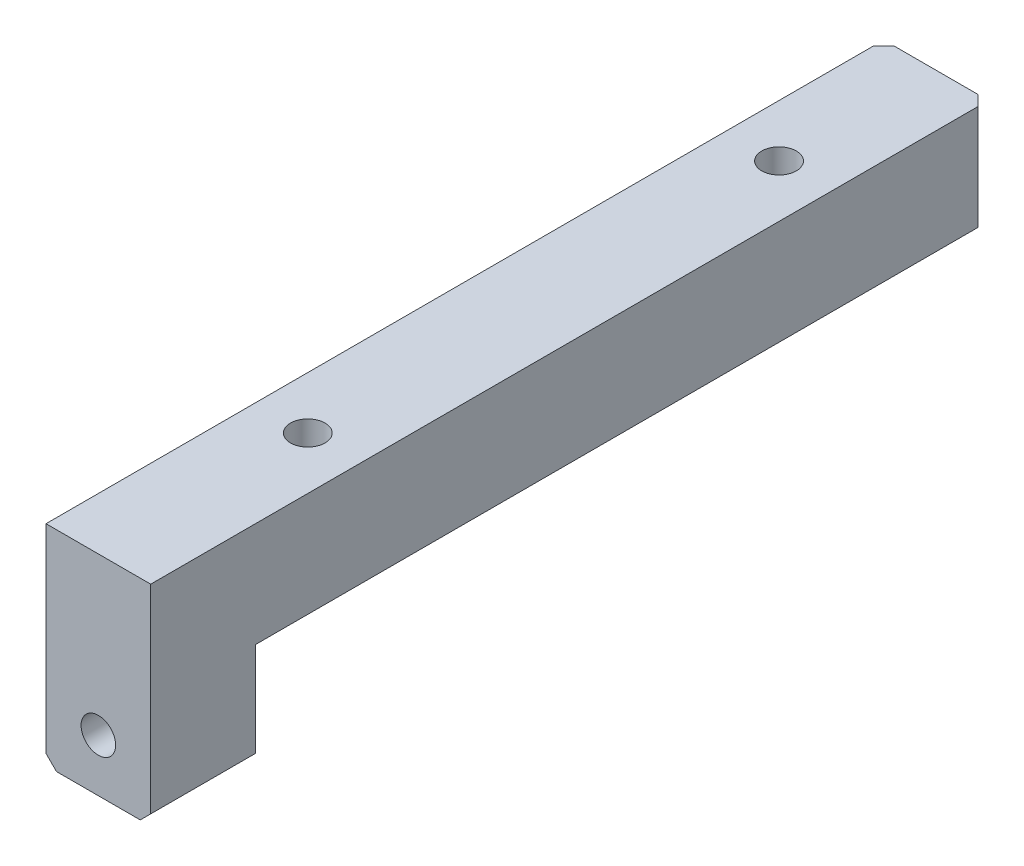
SolidWorks part; units mm, degrees
material "AL6061"
ref_plane "Front Plane" through (0, 0, 0) normal (0, 0, 1) x (1, 0, 0)
ref_plane "Top Plane" through (0, 0, 0) normal (0, 1, 0) x (1, 0, 0)
ref_plane "Right Plane" through (0, 0, 0) normal (1, 0, 0) x (0, 0, -1)
sketch "Sketch1" plane through (0, 0, 0) normal (1, 0, 0) x (0, 0, -1)
  line L1 (-40, -10) -> (40, -10)
  line L2 (-40, -10) -> (-40, 10)
  line L3 (-40, 10) -> (40, 10)
  line L4 (40, -10) -> (40, 10)
  line L5 (-40, -10) -> (40, 10) construction
  line L6 (-40, 10) -> (40, -10) construction
  point P0 (0, 0)
  dimension "D1" = 20
  dimension "D2" = 80
extrude "Boss-Extrude1" add sketch "Sketch1" along normal blind 10
sketch "Sketch3" plane through (0, 0, 0) normal (-1, 0, 0) x (0, 0, 1)
  line L0 (-40, 10) -> (40, 10) construction
  line L1 (-40, -10) -> (30, -10)
  line L2 (-40, -10) -> (-40, 0)
  line L3 (-40, 0) -> (30, 0)
  line L4 (30, -10) -> (30, 0)
  line L5 (40, 10) -> (40, -10) construction
  dimension "D1" = 10
  dimension "D2" = 10
extrude "Cut-Extrude1" cut sketch "Sketch3" against normal through all
hole_wizard "M4 Tapped Hole2" positions "Sketch6" profile "Sketch7" tap size "M4" standard "GB"
sketch "Sketch6" plane through (0, 0, 30) normal (0, 0, -1) x (-1, 0, 0)
  line L0 (-5, 0) -> (-5, -10) construction
  line L1 (-10, 0) -> (0, 0) construction
  line L2 (-10, -10) -> (0, -10) construction
  point P0 (-5, -5)
sketch "Sketch7" plane through (5, -5, 30) normal (1, 0, 0) x (0, 1, 0)
  line L0 (0, 0) -> (0, 11.0914)
  line L1 (0, 11.0914) -> (1.65, 10.1)
  line L2 (1.65, 10.1) -> (1.65, 0)
  line L5 (1.65, 0) -> (0, 0)
  line L10 (0, 11.0914) -> (-1.65, 10.1) construction
  line L11 (0, -6.35) -> (0, 107.95) construction
  dimension "螺纹孔钻头直径" = 3.3
  dimension "螺纹孔钻头深度" = 10.1
  dimension "导头角度" = 118
cosmetic thread "Cosmetic thread2"
chamfer "Chamfer1" distance 1 angle 45 4 edges at (0, 5, -40) (10, 5, -40) (10, -10, 35) (0, -10, 35)
hole_wizard "M4 Tapped Hole1" positions "Sketch8" profile "Sketch9" tap size "M4" standard "GB"
sketch "Sketch8" plane through (0, 10, 0) normal (0, 1, 0) x (1, 0, 0)
  line L0 (5, -40) -> (5, 40) construction
  line L1 (10, -40) -> (0, -40) construction
  line L2 (9, 40) -> (1, 40) construction
  point P0 (5, 25)
  point P16 (5, -20)
  dimension "D1" = 65
  dimension "D2" = 45
sketch "Sketch9" plane through (5, 10, -25) normal (1, 0, 0) x (0, 0, 1)
  line L0 (0, 0) -> (0, 11.0914)
  line L1 (0, 11.0914) -> (1.65, 10.1)
  line L2 (1.65, 10.1) -> (1.65, 0)
  line L5 (1.65, 0) -> (0, 0)
  line L10 (0, 11.0914) -> (-1.65, 10.1) construction
  line L11 (0, -6.35) -> (0, 107.95) construction
  dimension "螺纹孔钻头直径" = 3.3
  dimension "螺纹孔钻头深度" = 10.1
  dimension "导头角度" = 118
cosmetic thread "Cosmetic thread1"
cosmetic thread "Cosmetic thread3"
